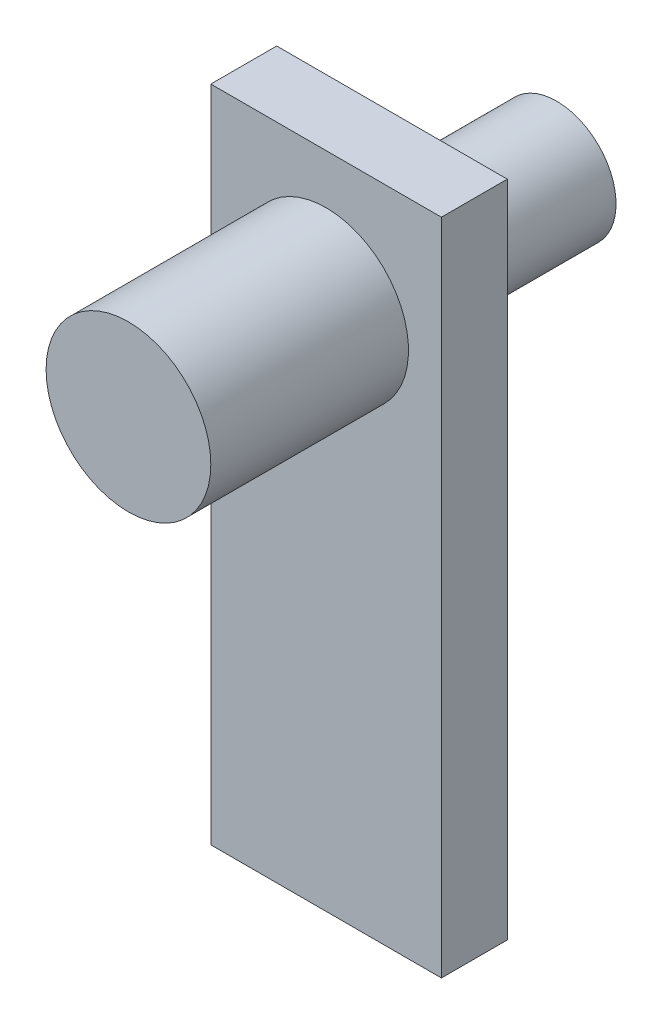
from build123d import *

# Parameters (mm, degrees)
SKETCH_1_W      = 35
SKETCH_1_H      = 100
EXTRUDE_1_DEPTH = 10
SKETCH_2_R      = 12.5
EXTRUDE_2_DEPTH = 30
SKETCH_3_R      = 9
EXTRUDE_3_DEPTH = 25


with BuildPart() as part:
    # 草图1 → 凸台-拉伸1 (new body)
    with BuildSketch(Plane.XY):
        Rectangle(SKETCH_1_W, SKETCH_1_H)
    extrude(amount=EXTRUDE_1_DEPTH)

    # 草图2 → 凸台-拉伸2 (add)
    with BuildSketch(Plane.XY.offset(10)):
        with Locations(Location((0, 30, 0), (0, 0, 180))):
            Circle(SKETCH_2_R)
    extrude(amount=EXTRUDE_2_DEPTH)

    # 草图3 → 凸台-拉伸3 (add)
    with BuildSketch(Plane(origin=(0, 0, 0), x_dir=(-1, 0, 0), z_dir=(0, 0, -1))):
        with Locations((0, 30)):
            Circle(SKETCH_3_R)
    extrude(amount=EXTRUDE_3_DEPTH)


solid = part.part
